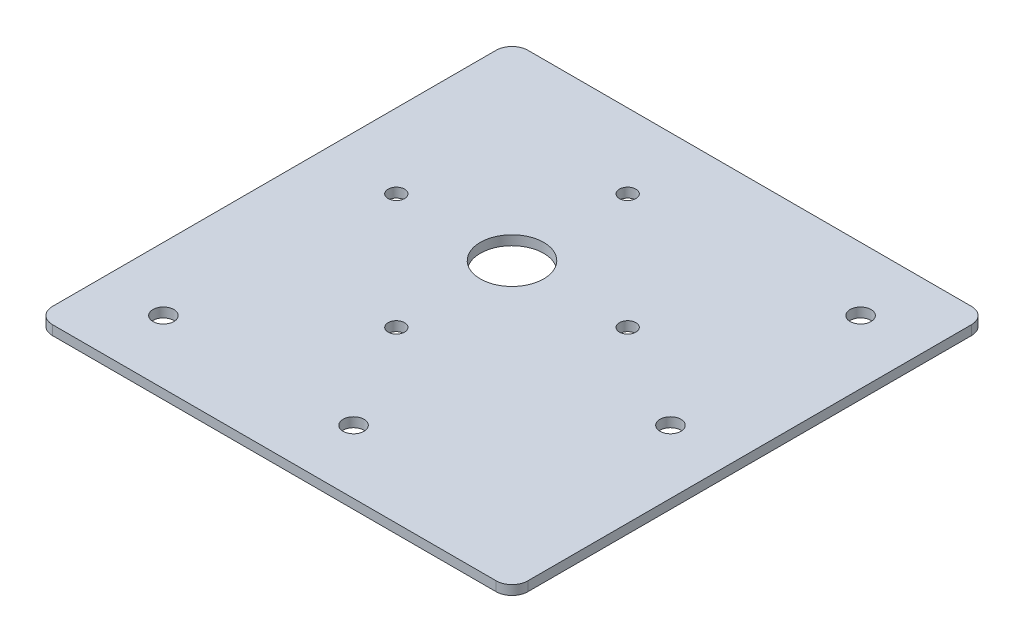
from build123d import *

# Parameters (mm, degrees)
SKETCH_1_W              = 150
SKETCH_1_H              = 150
EXTRUDE_1_DEPTH         = 3
HOLE_WIZARD_6_6_6_6_1_D = 6.6
FILLET_1_R              = 5
SKETCH_4_R              = 10
SKETCH_4_R_2            = 2.6
CUT_EXTRUDE_1_DEPTH     = 107.108435103


with BuildPart() as part:
    # 草图1 → 凸台-拉伸1 (new body)
    with BuildSketch(Plane(origin=(0, 0, 0), x_dir=(1, 0, 0), z_dir=(0, 1, 0))):
        Rectangle(SKETCH_1_W, SKETCH_1_H)
    extrude(amount=EXTRUDE_1_DEPTH)

    # Ø6.6 (6.6) 直径孔1 (through all)
    with Locations(Plane(origin=(0, 3, 0), x_dir=(-1, 0, 0), z_dir=(0, 1, 0))):
        with Locations((-55, 5), (-5, 55), (55, 55), (-55, -55)):
            Hole(HOLE_WIZARD_6_6_6_6_1_D / 2)

    # 圆角1
    fillet_1_edges = [part.edges().sort_by_distance(p)[0] for p in [
        (75, 1.5, 75),
        (-75, 1.5, 75),
        (-75, 1.5, -75),
        (75, 1.5, -75),
    ]]
    fillet(fillet_1_edges, radius=FILLET_1_R)

    # 草图4 → 切除-拉伸1 (cut, through all)
    with BuildSketch(Plane(origin=(0, 3, 0), x_dir=(1, 0, 0), z_dir=(0, 1, 0))):
        with Locations(Location((-15, 15, 0), (0, 0, 270))):
            Circle(SKETCH_4_R)
        with Locations(Location((-15, 51.5, 0), (0, 0, 270))):
            Circle(SKETCH_4_R_2)
        with Locations(Location((21.5, 15, 0), (0, 0, 270))):
            Circle(SKETCH_4_R_2)
        with Locations(Location((-15, -21.5, 0), (0, 0, 270))):
            Circle(SKETCH_4_R_2)
        with Locations(Location((-51.5, 15, 0), (0, 0, 270))):
            Circle(SKETCH_4_R_2)
    extrude(amount=-CUT_EXTRUDE_1_DEPTH, mode=Mode.SUBTRACT)


solid = part.part
